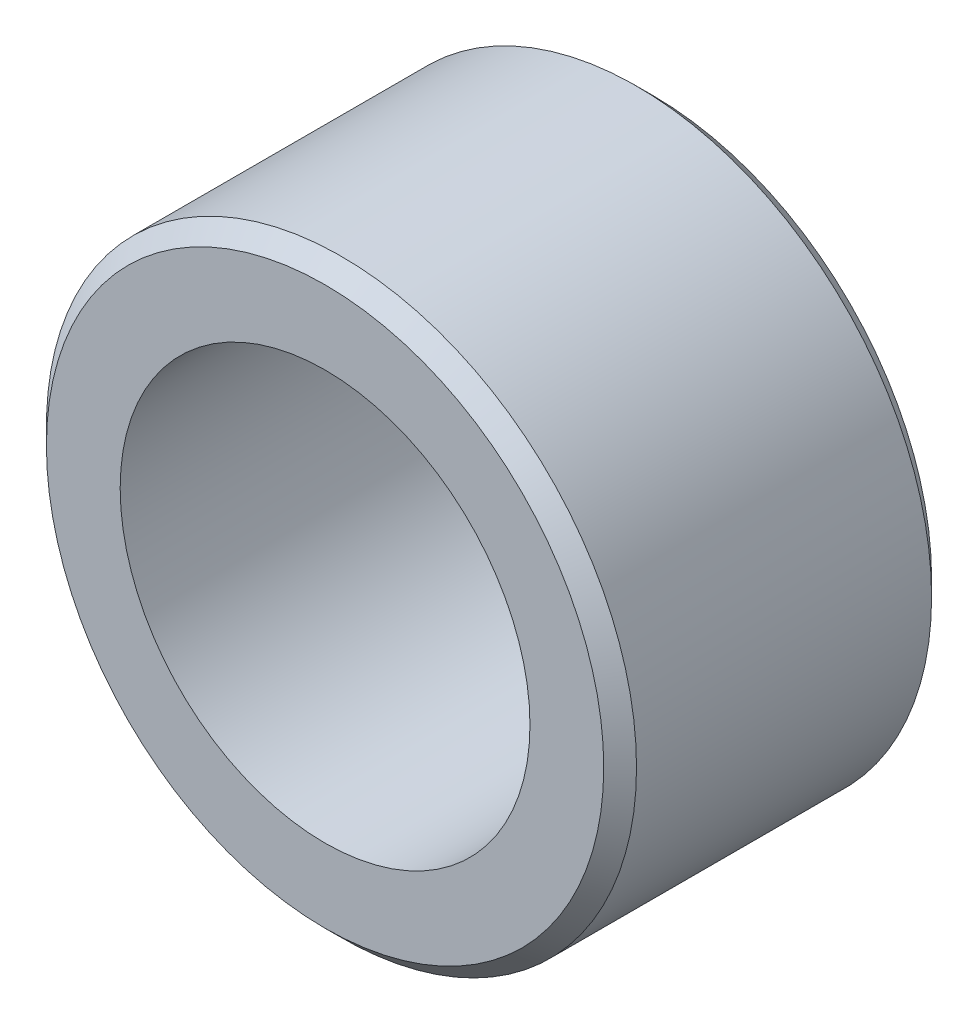
from build123d import *

# Parameters (mm, degrees)
SKETCH1_R           = 9
SKETCH1_R_2         = 6.25
BOSS_EXTRUDE1_DEPTH = 10
CHAMFER1_SIZE       = 0.5


with BuildPart() as part:
    # Sketch1 → Boss-Extrude1 (new body)
    with BuildSketch(Plane.XY):
        Circle(SKETCH1_R)
        Circle(SKETCH1_R_2, mode=Mode.SUBTRACT)
    extrude(amount=BOSS_EXTRUDE1_DEPTH)

    # Chamfer1
    chamfer1_edges = [part.edges().sort_by_distance(p)[0] for p in [
        (-9, 0, 0),
        (-9, 0, 10),
    ]]
    chamfer(chamfer1_edges, length=CHAMFER1_SIZE)


solid = part.part
